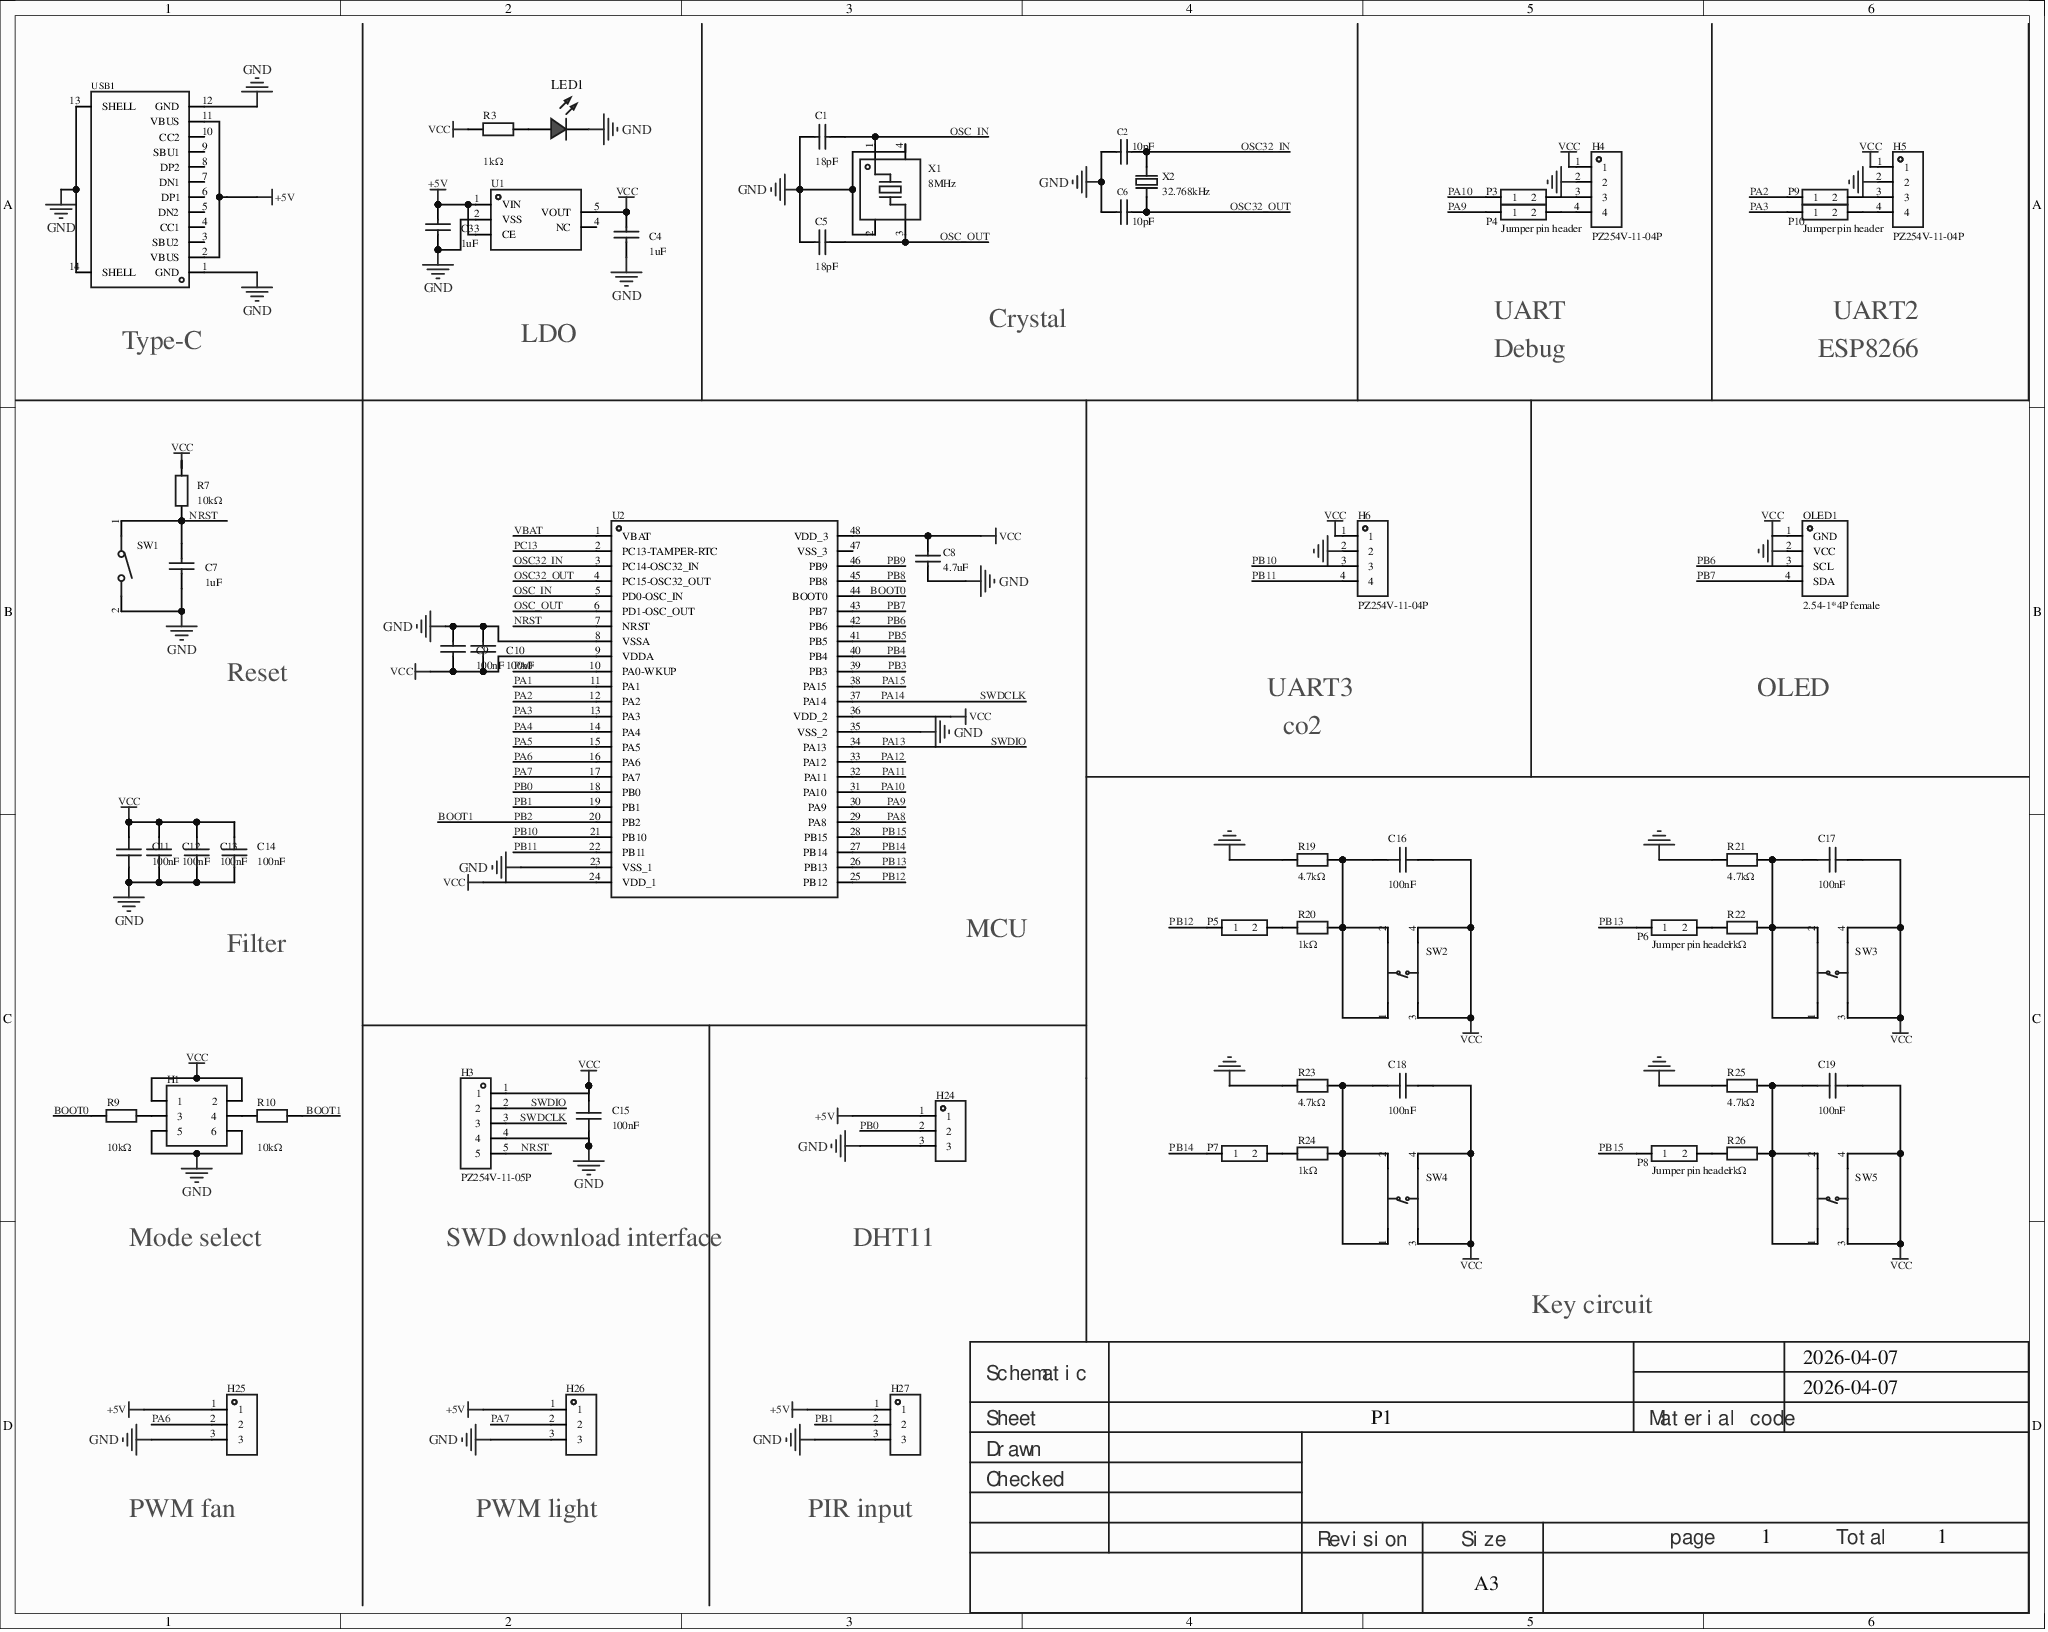
[diagram p0: MISC61607-3.schdoc]
# Altium project MISC61607-2.PrjPcb
1 sheet, 60 parts. Net scope: global (net labels, ports and power ports of the same name join across sheets).
Board file: MISC61607.pcbdoc

## Sheet MISC61607-3.schdoc
size 344 x 274 mm; Version: V1.0; @Project Name: MISC61607; @Page Count: 1; @Update Date: 2026-04-07; @Create Date: 2026-04-07; @Schematic Name: MISC61607; @Page No: 1; @Board Name: MISC61607; @Create Time: 19:36:59; @Update Time: 19:36:59

### Parts
C1  value 18pF  [C0603]  (hidden comment: FCC0603N180J500CT)
C2  value 10pF  [C0603]  (hidden comment: CL10C100JB8NNNC)
C3  value 1uF  [C0603]  (hidden comment: CL05A105KP5NNNC)
C4  value 1uF  [C0603]  (hidden comment: CL05A105KQ5NNNC)
C5  value 18pF  [C0603]  (hidden comment: FCC0603N180J500CT)
C6  value 10pF  [C0603]  (hidden comment: CL10C100JB8NNNC)
C7  value 1uF  [C0603]  (hidden comment: CGA0603X5R105K500JT)
C8  value 4.7uF  [C0603]  (hidden comment: CL10A475KO8NNNC)
C9  value 100nF  [C0603]  (hidden comment: CC0603KRX7R9BB104)
C10  value 100nF  [C0603]  (hidden comment: CC0603KRX7R9BB104)
C11  value 100nF  [C0603]  (hidden comment: CC0603KRX7R9BB104)
C12  value 100nF  [C0603]  (hidden comment: CC0603KRX7R9BB104)
C13  value 100nF  [C0603]  (hidden comment: CC0603KRX7R9BB104)
C14  value 100nF  [C0603]  (hidden comment: CC0603KRX7R9BB104)
C15  value 100nF  [C0603]  (hidden comment: CC0603KRX7R9BB104)
C16  100nF  [C0603]
C17  100nF  [C0603]
C18  100nF  [C0603]
C19  100nF  [C0603]
H1  (no value)  [HDR-TH_6P-P2.54-V-R2-C3-S2.54_A2541WV-2X3P]
H3  PZ254V-11-05P  [HDR-TH_5P-P2.54-V-M]
H4  PZ254V-11-04P  [HDR-TH_4P-P2.54-V-M]
H5  PZ254V-11-04P  [HDR-TH_4P-P2.54-V-M]
H6  PZ254V-11-04P  [HDR-TH_4P-P2.54-V-M]
H24  HC-PM254-8.5H-1x3PW-02A  [HDR-TH_3P-P2.54_HC-PM254-8.5H-1X3PW]  (value not drawn)
H25  HC-PM254-8.5H-1x3PW-02A  [HDR-TH_3P-P2.54_HC-PM254-8.5H-1X3PW]  (value not drawn)
H26  HC-PM254-8.5H-1x3PW-02A  [HDR-TH_3P-P2.54_HC-PM254-8.5H-1X3PW]  (value not drawn)
H27  HC-PM254-8.5H-1x3PW-02A  [HDR-TH_3P-P2.54_HC-PM254-8.5H-1X3PW]  (value not drawn)
LED1  LED_0402-R  [LED_0402]  (value not drawn)
OLED1  2.54-1*4P female  [HDR-TH_4P-P2.54-V-F]
P3  Jumper pin header  [2P排针]  (value not drawn)
P4  Jumper pin header  [2P排针]
P5  Jumper pin header  [2P排针]  (value not drawn)
P6  Jumper pin header  [2P排针]
P7  Jumper pin header  [2P排针]  (value not drawn)
P8  Jumper pin header  [2P排针]
P9  Jumper pin header  [2P排针]  (value not drawn)
P10  Jumper pin header  [2P排针]
R3  value 1kΩ  [R0603]  (hidden comment: 0603WAF1001T5E)
R7  value 10kΩ  [R0603]  (hidden comment: 0603WAF1002T5E)
R9  value 10kΩ  [R0603]  (hidden comment: 0603WAF1002T5E)
R10  value 10kΩ  [R0603]  (hidden comment: 0603WAF1002T5E)
R19  4.7kΩ  [R0603]
R20  1kΩ  [R0603]
R21  4.7kΩ  [R0603]
R22  1kΩ  [R0603]
R23  4.7kΩ  [R0603]
R24  1kΩ  [R0603]
R25  4.7kΩ  [R0603]
R26  1kΩ  [R0603]
SW1  TS-1088-AR02016  [SW-SMD_L3.9-W3.0-P4.45]  (value not drawn)
SW2  TS665CJ  [SW-TH_4P-L6.0-W6.0-P4.50-LS6.5]  (value not drawn)
SW3  TS665CJ  [SW-TH_4P-L6.0-W6.0-P4.50-LS6.5]  (value not drawn)
SW4  TS665CJ  [SW-TH_4P-L6.0-W6.0-P4.50-LS6.5]  (value not drawn)
SW5  TS665CJ  [SW-TH_4P-L6.0-W6.0-P4.50-LS6.5]  (value not drawn)
U1  ME6211C33M5G-N  [SOT-23-5_L3.0-W1.7-P0.95-LS2.8-BL]  (value not drawn)
U2  STM32F103C8T6  [LQFP-48_L7.0-W7.0-P0.50-LS9.0-BL]  (value not drawn)
USB1  TYPE-C 16PIN 2MD(073)  [USB-C-SMD_TYPE-C-6PIN-2MD-073]  (value not drawn)
X1  8MHz  [OSC-SMD_4P-L3.2-W2.5-BL]
X2  value 32.768kHz  [CRYSTAL-SMD_L3.2-W1.5-1]  (hidden comment: Q13FC13500049)

### Nets
+5V: C3.2 H24.1 H25.1 H26.1 H27.1 U1.1(VIN) U1.3(CE) USB1.2(VBUS) USB1.11(VBUS)
GND: C1.2 C2.1 C3.1 C4.1 C5.2 C6.1 C7.2 C8.1 C9.2 C10.2 C11.1 C12.1 C13.1 C14.1 C15.1 H1.5 H1.6 H3.4 H4.2 H5.2 H6.2 H24.3 H25.3 H26.3 H27.3 LED1.1(C) OLED1.2(VCC) R19.1 R21.1 R23.1 R25.1 SW1.2 U1.2(VSS) U2.8(VSSA) U2.23(VSS_1) U2.35(VSS_2) USB1.1(GND) USB1.12(GND) USB1.13(SHELL) USB1.14(SHELL) X1.2(GND) X1.4(GND)
VCC: C4.2 C8.2 C9.1 C10.1 C11.2 C12.2 C13.2 C14.2 C15.2 C16.2 C17.2 C18.2 C19.2 H1.1 H1.2 H3.1 H4.1 H5.1 H6.1 OLED1.1(GND) R3.1 R7.2 SW2.3(C) SW2.4(D) SW3.3(C) SW3.4(D) SW4.3(C) SW4.4(D) SW5.3(C) SW5.4(D) U1.5(VOUT) U2.9(VDDA) U2.24(VDD_1) U2.36(VDD_2) U2.48(VDD_3)
BOOT0: R9.1 U2.44(BOOT0)
BOOT1: R10.2 U2.20(PB2)  [also labelled PB2]
NRST: C7.1 H3.5 R7.1 SW1.1 U2.7(NRST)
OSC32_IN: C2.2 U2.3(PC14-OSC32_IN) X2.2
OSC32_OUT: C6.2 U2.4(PC15-OSC32_OUT) X2.1
OSC_IN: C1.1 U2.5(PD0-OSC_IN) X1.1
OSC_OUT: C5.1 U2.6(PD1-OSC_OUT) X1.3
PA0: U2.10(PA0-WKUP)
PA1: U2.11(PA1)
PA2: P9.1 U2.12(PA2)
PA3: P10.1 U2.13(PA3)
PA4: U2.14(PA4)
PA5: U2.15(PA5)
PA6: H25.2 U2.16(PA6)
PA7: H26.2 U2.17(PA7)
PA8: U2.29(PA8)
PA9: P4.1 U2.30(PA9)
PA10: P3.1 U2.31(PA10)
PA11: U2.32(PA11)
PA12: U2.33(PA12)
PA13: H3.2 U2.34(PA13)  [also labelled SWDIO]
PA14: H3.3 U2.37(PA14)  [also labelled SWDCLK]
PA15: U2.38(PA15)
PB0: H24.2 U2.18(PB0)
PB1: H27.2 U2.19(PB1)
PB3: U2.39(PB3)
PB4: U2.40(PB4)
PB5: U2.41(PB5)
PB6: OLED1.3(SCL) U2.42(PB6)
PB7: OLED1.4(SDA) U2.43(PB7)
PB8: U2.45(PB8)
PB9: U2.46(PB9)
PB10: H6.3 U2.21(PB10)
PB11: H6.4 U2.22(PB11)
PB12: P5.1 U2.25(PB12)
PB13: P6.1 U2.26(PB13)
PB14: P7.1 U2.27(PB14)
PB15: P8.1 U2.28(PB15)
PC13: U2.2(PC13-TAMPER-RTC)
VBAT: U2.1(VBAT)
NetC16_1: C16.1 R19.2 R20.2 SW2.1(A) SW2.2(B)
NetC17_1: C17.1 R21.2 R22.2 SW3.1(A) SW3.2(B)
NetC18_1: C18.1 R23.2 R24.2 SW4.1(A) SW4.2(B)
NetC19_1: C19.1 R25.2 R26.2 SW5.1(A) SW5.2(B)
NetH1_3: H1.3 R9.2
NetH1_4: H1.4 R10.1
NetH4_3: H4.3 P3.2
NetH4_4: H4.4 P4.2
NetH5_3: H5.3 P9.2
NetH5_4: H5.4 P10.2
NetLED1_2: LED1.2(A) R3.2
NetP5_2: P5.2 R20.1
NetP6_2: P6.2 R22.1
NetP7_2: P7.2 R24.1
NetP8_2: P8.2 R26.1

Not connected (* = marked no-connect by the designer): U1 4(NC)*; U2 47(VSS_3); USB1 3(SBU2)* 4(CC1) 5(DN2) 6(DP1) 7(DN1) 8(DP2) 9(SBU1)* 10(CC2)

### Notes on the sheet
- (near USB1) Type-C
- LDO
- Crystal
- UART
- Debug
- ESP8266
- UART2
- Reset
- UART3
- co2
- OLED
- Filter
- MCU
- Mode select
- SWD download interface
- DHT11
- Key circuit
- (near H25) PWM fan
- (near H26) PWM light
- (near H27) PIR input
- 2026-04-07
- Schematic
- Sheet
- P1
- Material code
- Checked
- Drawn
- Revision
- Size
- A3
- page
- 1
- Total

### Library data of the parts
C1 C5 = FCC0603N180J500CT: Capacitance:18pF; tolerance:±5%; rated voltage:50V; temperature coefficient:C0G;; Manufacturer: FOJAN(富捷); Symbol: 0402CG180J500NT; AddInBom: yes; ModelId: ac125912035d415993ca9572d50418b1; ModelName: C0603_L1.6-W0.8-H0.8; ModelTransform: 62.992,31.496,0,0,0,0,0,0,0; Tolerance: ±5%; Voltage Rating: 50V; Temperature Coefficient: C0G; Device: FCC0603N180J500CT; Supplier: LCSC; Manufacturer Part: FCC0603N180J500CT; Supplier Part: C5137620; JLCPCB Part Class: Extended Part; LCSC Part Name: 18pF ±5% 50V; Supplier Footprint: 0603; Datasheet: https://atta.szlcsc.com/upload/public/pdf/source/20220818/0EB3B7FB2F5648AC16609637FBA7DABE.pdf; ConvertToPcb: yes; FootprintName: C0603
C2 C6 = CL10C100JB8NNNC: Capacitance:10pF; tolerance:±5%; rated voltage:50V; temperature coefficient:C0G;; Manufacturer: SAMSUNG(三星); Symbol: 0402CG100J500NT; AddInBom: yes; ModelId: ac125912035d415993ca9572d50418b1; ModelName: C0603_L1.6-W0.8-H0.8; ModelTransform: 62.992,31.496,0,0,0,0,0,0,0; Tolerance: ±5%; Voltage Rating: 50V; Temperature Coefficient: C0G; Device: CL10C100JB8NNNC; Supplier: LCSC; Manufacturer Part: CL10C100JB8NNNC; Capacitance: 10pF; Supplier Part: C1634; JLCPCB Part Class: Basic Part; LCSC Part Name: 10pF ±5% 50V; Supplier Footprint: 0603; Datasheet: https://item.szlcsc.com/datasheet/CL10C100JB8NNNC/1986.html; ConvertToPcb: yes; FootprintName: C0603
C3 = CL05A105KP5NNNC: Capacitance:1uF; tolerance:±10%; rated voltage:10V; dielectric (temperature coefficient):X5R;; Manufacturer: SAMSUNG(三星); AddInBom: yes; ModelId: 36a51122f27c49738f86b3bfa98863e0; ModelName: C0402_L1.0-W0.5-H0.5; ModelTransform: 39.37,19.685,0,0,0,0,0,0,0; Tolerance: ±10%; Voltage Rated: 10V; Temperature Coefficient: X5R; Symbol: CL05A105KP5NNNC; Device: CL05A105KP5NNNC; Supplier: LCSC; Manufacturer Part: CL05A105KP5NNNC; Supplier Part: C14445; JLCPCB Part Class: Extended library; LCSC Part Name: 1uF ±10% 10V; Supplier Footprint: 0402; Datasheet: https://atta.szlcsc.com/upload/public/pdf/source/20160218/1457707763339.pdf; ConvertToPcb: yes; FootprintName: C0603
C4 = CL05A105KQ5NNNC: Capacitance:1uF; tolerance:±10%; rated voltage:6.3V; dielectric (temperature coefficient):X5R;; Manufacturer: SAMSUNG(三星); AddInBom: yes; ModelId: 36a51122f27c49738f86b3bfa98863e0; ModelName: C0402_L1.0-W0.5-H0.5; ModelTransform: 39.37,19.685,0,0,0,0,0,0,0; Tolerance: ±10%; Voltage Rated: 6.3V; Temperature Coefficient: X5R; Symbol: CL05A105KQ5NNNC; Device: CL05A105KQ5NNNC; Supplier: LCSC; Manufacturer Part: CL05A105KQ5NNNC; Supplier Part: C107372; JLCPCB Part Class: Extended library; LCSC Part Name: 1uF ±10% 6.3V; Supplier Footprint: 0402; Datasheet: https://atta.szlcsc.com/upload/public/pdf/source/20160218/1457707763339.pdf; ConvertToPcb: yes; FootprintName: C0603
C7 = CGA0603X5R105K500JT: Capacitance:1uF; tolerance:±10%; rated voltage:50V; temperature coefficient:X5R;; Manufacturer: HRE(芯声); Symbol: CL05A105KQ5NNNC; AddInBom: yes; ModelId: ac125912035d415993ca9572d50418b1; ModelName: C0603_L1.6-W0.8-H0.8; ModelTransform: 62.992,31.496,0,0,0,0,0,0,0; Tolerance: ±10%; Voltage Rating: 50V; Temperature Coefficient: X5R; Device: CGA0603X5R105K500JT; Supplier: LCSC; Manufacturer Part: CGA0603X5R105K500JT; Supplier Part: C6119852; JLCPCB Part Class: Extended Part; LCSC Part Name: 1uF ±10% 50V; Supplier Footprint: 0603; ConvertToPcb: yes; FootprintName: C0603
C8 = CL10A475KO8NNNC: Capacitance:4.7uF; tolerance:±10%; rated voltage:16V; temperature coefficient:X5R;; Manufacturer: SAMSUNG(三星); Symbol: CL05A475MP5NRNC; AddInBom: yes; ModelId: ac125912035d415993ca9572d50418b1; ModelName: C0603_L1.6-W0.8-H0.8; ModelTransform: 62.992,31.496,0,0,0,0,0,0,0; Tolerance: ±10%; Voltage Rating: 16V; Temperature Coefficient: X5R; Device: CL10A475KO8NNNC; Supplier: LCSC; Manufacturer Part: CL10A475KO8NNNC; Supplier Part: C19666; JLCPCB Part Class: Basic Part; LCSC Part Name: 4.7uF ±10% 16V; Supplier Footprint: 0603; Datasheet: https://item.szlcsc.com/datasheet/CL10A475KO8NNNC/20375.html; ConvertToPcb: yes; FootprintName: C0603
C9 = CC0603KRX7R9BB104: Capacitance:100nF; tolerance:±10%; rated voltage:50V; temperature coefficient:X7R;; Manufacturer: YAGEO(国巨); Symbol: CC0402KRX7R9BB103; AddInBom: yes; ModelId: ac125912035d415993ca9572d50418b1; ModelName: C0603_L1.6-W0.8-H0.8; ModelTransform: 62.992,31.496,0,0,0,0,0,0,0; Tolerance: ±10%; Voltage Rating: 50V; Temperature Coefficient: X7R; Device: CC0603KRX7R9BB104; Supplier: LCSC; Manufacturer Part: CC0603KRX7R9BB104; Supplier Part: C14663; JLCPCB Part Class: Basic Part; LCSC Part Name: 100nF ±10% 50V; Supplier Footprint: 0603; Datasheet: https://item.szlcsc.com/datasheet/CC0603KRX7R9BB104/15331.html; ConvertToPcb: yes; FootprintName: C0603
C10 = CC0603KRX7R9BB104: Capacitance:100nF; tolerance:±10%; rated voltage:50V; temperature coefficient:X7R;; Manufacturer: YAGEO(国巨); Symbol: CL05A105KP5NNNC; AddInBom: yes; ModelId: ac125912035d415993ca9572d50418b1; ModelName: C0603_L1.6-W0.8-H0.8; ModelTransform: 62.992,31.496,0,0,0,0,0,0,0; Tolerance: ±10%; Voltage Rating: 50V; Temperature Coefficient: X7R; Device: CC0603KRX7R9BB104; Supplier: LCSC; Manufacturer Part: CC0603KRX7R9BB104; Supplier Part: C14663; JLCPCB Part Class: Basic Part; LCSC Part Name: 100nF ±10% 50V; Supplier Footprint: 0603; Datasheet: https://item.szlcsc.com/datasheet/CC0603KRX7R9BB104/15331.html; ConvertToPcb: yes; FootprintName: C0603
C11-C15 = CC0603KRX7R9BB104: Capacitance:100nF; tolerance:±10%; rated voltage:50V; temperature coefficient:X7R;; Manufacturer: YAGEO(国巨); Symbol: CC0402KRX7R7BB104; AddInBom: yes; ModelId: ac125912035d415993ca9572d50418b1; ModelName: C0603_L1.6-W0.8-H0.8; ModelTransform: 62.992,31.496,0,0,0,0,0,0,0; Tolerance: ±10%; Voltage Rating: 50V; Temperature Coefficient: X7R; Device: CC0603KRX7R9BB104; Supplier: LCSC; Manufacturer Part: CC0603KRX7R9BB104; Supplier Part: C14663; JLCPCB Part Class: Basic Part; LCSC Part Name: 100nF ±10% 50V; Supplier Footprint: 0603; Datasheet: https://item.szlcsc.com/datasheet/CC0603KRX7R9BB104/15331.html; ConvertToPcb: yes; FootprintName: C0603
C16-C19 = CGA0603X7R104K500JT: Capacitance:100nF; tolerance:±10%; rated voltage:50V; temperature coefficient:X7R;; Manufacturer: HRE(芯声); AddInBom: yes; ModelId: ac125912035d415993ca9572d50418b1; ModelName: C0603_L1.6-W0.8-H0.8; ModelTransform: 62.992,31.496,0,0,0,0,0,0,0; Tolerance: ±10%; Voltage Rating: 50V; Temperature Coefficient: X7R; Symbol: CGA0603X7R104K500JT; Device: CGA0603X7R104K500JT; LCSC Part Name: 100nF ±10% 50V; SupplierPart: C6119867; ManufacturerPart: CGA0603X7R104K500JT; Supplier Footprint: 0603; Datasheet: https://atta.szlcsc.com/upload/public/pdf/source/20250103/C44077DA9E7B3EFAE02F22B6D3D1CBC9.pdf; Supplier: LCSC; ConvertToPcb: yes; FootprintName: C0603; Value: 100nF
H1 = HDR-M_2.54_2x3: Symbol: HDR-M-2.54_2x3; ConvertToPcb: yes; ModelId: fd1b55b786fb415ca65c4187088147b7; ModelName: HDR2.54-M-LI-2x3P; ModelTransform: 299.9994,200,0,0,0,0,0,0,-118.11; Device: HDR-M_2.54_2x3; AddInBom: yes; SupplierPart: C402781; Supplier Footprint: 插件,P=2.54mm; FootprintName: HDR-TH_6P-P2.54-V-R2-C3-S2.54_A2541WV-2X3P
H3 = PZ254V-11-05P: Pin structure:1x5P; pitch:2.54mm; row spacing:-; round/square pin:square pin; mounting:through-hole; rows:single row; total PIN count:5P; rated current:-; rated voltage:-; mating pin length:6mm; plastic height:2.5mm; tail length:3mm; contact material:brass; contact plating:-; operating temperature:-40℃~+105℃; colour:black;; Manufacturer: XFCN(兴飞); AddInBom: yes; ModelId: 47d466e4a34f4fc5bc626cf773a24dd5; ModelName: HDR-TH_5P-P2.54-M-LI-1X5P; ModelTransform: 499.999,100,0,0,0,0,0,0,-118.11; Pin Structure: 1x5P; Pitch: 2.54mm; Symbol: PZ254V-11-05P; Device: PZ254V-11-05P; LCSC Part Name: 1x5P 间距:2.54mm 方针 直插; SupplierPart: C492404; ManufacturerPart: PZ254V-11-05P; Supplier Footprint: 插件,P=2.54mm; JLCPCB Part Class: Extended library; Datasheet: https://atta.szlcsc.com/upload/public/pdf/source/20200309/C492404_E51533260F8710EFF5D4617281164C1D.pdf; Supplier: LCSC; ConvertToPcb: yes; FootprintName: HDR-TH_5P-P2.54-V-M; Row Spacing: -; Circluar Pins/Square Pins: Square pin; Mounting Type: Through-hole; Number of Rows: Single row; Number of Pins: 5P; Current Rating: -; Voltage Rating (Max): -; Length of Mating Pin: 6mm; Insulation Height: 2.5mm; Length of End Connection Pin: 3mm; Contact Material: Brass; Contact Plating: -; Operating Temperature: -40℃~+105℃; Color: Black
H4-H6 = PZ254V-11-04P: Pin structure:1x4P; pitch:2.54mm; row spacing:-; round/square pin:square pin; mounting:through-hole; rows:single row; total PIN count:4P; rated current:3A; rated voltage:250V; mating pin length:6mm; plastic height:2.5mm; tail length:3mm; contact material:-; operating temperature:-40℃~+105℃; colour:black;; Manufacturer: XFCN(兴飞); Symbol: PZ254V-11-04P_C2691448; AddInBom: yes; ModelId: 112f4d05e8d64e99ab9a333894bea4f9; ModelName: HDR-TH_4P-P2.54-M-LI-1X4P; ModelTransform: 399.999,104.7242,0,0,0,0,0,0,-118.11; Pin Structure: 1x4P; Pitch: 2.54mm; Current Rating: 3A; Voltage Rating (Max): 250V; Device: PZ254V-11-04P; LCSC Part Name: 1x4P 间距:2.54mm 方针 直插; SupplierPart: C2691448; ManufacturerPart: PZ254V-11-04P; Supplier Footprint: 插件,P=2.54mm; JLCPCB Part Class: Extended library; Datasheet: https://item.szlcsc.com/datasheet/PZ254V-11-04P/2801085.html; Supplier: LCSC; ConvertToPcb: yes; FootprintName: HDR-TH_4P-P2.54-V-M; Row Spacing: -; Circluar Pins/Square Pins: Square pin; Mounting Type: Through-hole; Number of Rows: Single row; Number of Pins: 4P; Length of Mating Pin: 6mm; Insulation Height: 2.5mm; Length of End Connection Pin: 3mm; Contact Material: -; Operating Temperature: -40℃~+105℃; Color: Black
H24-H27 = HC-PM254-8.5H-1x3PW-02A: Socket structure:1x3P; pitch:2.54mm; row spacing:-; round/square hole:square hole; mounting:bent (right-angle); rows:single row; total hole count:3P; rated current:3A; rated voltage:-; socket direction:side; plastic height:2.5mm; contact material:brass; contact plating:gold; operating temperature:-40℃~+105℃;; Manufacturer: HC(虹成电子); AddInBom: yes; ModelId: e14a0b847ce14913bcceafd4aa6783c3; ModelTransform: 320.078,397.637,0,0,0,0,0,-194.133,-125.984; Holes Structure: 1x3P; Pitch: 2.54mm; Number of Positions: 3P; Current Rating: 3A; Holes Direction: Side; PIN Length: 3mm; Symbol: HC-PM254-8.5H-1X3PW; Device: HC-PM254-8.5H-1x3PW-02A; LCSC Part Name: 间距2.54mm 1x3Pin 弯插 PC3.2 PB10.2 H8.5; SupplierPart: C22373927; ManufacturerPart: HC-PM254-8.5H-1x3PW-02A; Supplier Footprint: 弯插,P=2.54mm; Datasheet: https://atta.szlcsc.com/upload/public/pdf/source/20250106/76C6231410311B19092B3A33DDCC33AF.pdf; Supplier: LCSC; ConvertToPcb: yes; FootprintName: HDR-TH_3P-P2.54_HC-PM254-8.5H-1X3PW; ModelName: HDR-TH_3P-P2.54_HC-PM254-8.5H-1X3PW; Row Spacing: -; Circular Hole / Square Hole: Square hole; Mounting Type: Bent (right-angle); Number of Rows: Single row; Voltage Rating (Max): -; Insulation Height: 2.5mm; Contact Material: Brass; Contact Plating: Gold; Operating Temperature: -40℃~+105℃; Supplementary Features: -
LED1 = LED_0402-R: Symbol: LED_R; Convert to PCB: yes; 3D Model: ff479c6f784e45d5abe8f8ff531b4a70; 3D Model Transform: 39.4,19.7,15.76,180,0,0,0,0,0; ModelName: LED0402-RD_ORANGE; Device: LED_0402-R; Add into BOM: yes; Supplier Footprint: 0402; FootprintName: LED_0402
OLED1 = 2.54-1*4P母: Socket structure:1x4P; pitch:2.54mm; row spacing:-; round/square hole:square hole; mounting:through-hole; rows:single row; total hole count:4P; rated current:3A; rated voltage:-; socket direction:top; plastic height:-; contact material:bronze; contact plating:-; operating temperature:-40℃~+105℃;; Manufacturer: BOOMELE(博穆精密); Symbol: HS96L03W2C03; AddInBom: yes; ModelId: d187812051054f85879fcaa51a310d8e; ModelTransform: 419.6842,98.464,0,0,0,0,0,0,-118.11; Holes Structure: 1x4P; Pitch: 2.54mm; Number of Positions: 4P; Current Rating: 3A; Holes Direction: Top; Device: 2.54-1*4P female; LCSC Part Name: 间距:2.54mm 1x4P 直插; SupplierPart: C2718488; ManufacturerPart: 2.54-1*4P母; Supplier Footprint: 插件,P=2.54mm; JLCPCB Part Class: Extended Part; Datasheet: https://item.szlcsc.com/datasheet/2.54-1*4P%25E6%25AF%258D/2834502.html; Supplier: LCSC; ConvertToPcb: yes; FootprintName: HDR-TH_4P-P2.54-V-F; ModelName: HDR-TH_4P-P2.54-V-F; Row Spacing: -; Circular Hole / Square Hole: Square hole; Mounting Type: Through-hole; Number of Rows: Single row; Voltage Rating (Max): -; Insulation Height: -; Contact Material: Bronze; Contact Plating: -; Operating Temperature: -40℃~+105℃
P3-P10 = 跳线排针-1.27mm-1×2P: AddInBom: yes; Device: 跳线排针-1.27mm-1×2P; 物料号: *; 名称: Jumper pin header; 封装: 1.27mm-1×2P; 规格: 1.27mm-1×2P; 型号: *; 替换型号: *; 厂商: *; Footprint Name: 跳线排针-1.27mm-1×2P; ConvertToPcb: yes; SymbolName: 跳线排针-1.27mm-1×2P
R3 = 0603WAF1001T5E: Resistor type:thick film resistor; resistance:1kΩ; tolerance:±1%; power:100mW; max working voltage:75V; temperature coefficient:±100ppm/℃;; Manufacturer: UNI-ROYAL(厚声); Symbol: 0402WGF1001TCE; AddInBom: yes; ModelId: fc143cca1e79419f9cd78b61e9279f08; ModelTransform: 31.8897,63.7794,0,90,0,0,0,0,0; Tolerance: ±1%; Power(Watts): 100mW; Overload Voltage (Max): 75V; JLCPCB Part Class: Basic Part; Device: 0603WAF1001T5E; Supplier: LCSC; Manufacturer Part: 0603WAF1001T5E; Supplier Part: C21190; LCSC Part Name: 1kΩ ±1% 100mW 厚膜电阻; Supplier Footprint: 0603; Datasheet: https://atta.szlcsc.com/upload/public/pdf/source/20200306/C422600_1E6D84923E4A46A82E41ADD87F860B5C.pdf; ConvertToPcb: yes; FootprintName: R0603; ModelName: R0603; Type: Thick film resistor; Temperature Coefficient: ±100ppm/℃; Operating Temperature Range: -55℃~+155℃
R7 R9 R10 = 0603WAF1002T5E: Resistor type:thick film resistor; resistance:10kΩ; tolerance:±1%; power:100mW; working voltage:75V; temperature coefficient:±100ppm/℃;; Manufacturer: UNI-ROYAL(厚声); Symbol: RC0402FR-0710KL; AddInBom: yes; ModelId: fc143cca1e79419f9cd78b61e9279f08; ModelTransform: 31.8897,63.7794,0,90,0,0,0,0,0; Tolerance: ±1%; Power(Watts): 100mW; Voltage-Supply(Max): 75V; Device: 0603WAF1002T5E; LCSC Part Name: 厚膜电阻 10kΩ ±1% 100mW; SupplierPart: C25804; ManufacturerPart: 0603WAF1002T5E; Supplier Footprint: 0603; JLCPCB Part Class: Basic Part; Datasheet: https://item.szlcsc.com/datasheet/0603WAF1002T5E/26547.html; Supplier: LCSC; ConvertToPcb: yes; FootprintName: R0603; ModelName: R0603; Type: Thick film resistor; Temperature Coefficient: ±100ppm/℃; Operating Temperature: -55℃~+155℃
R19 R21 R23 R25 = 0603WAF4701T5E: Resistor type:thick film resistor; resistance:4.7kΩ; tolerance:±1%; power:100mW; working voltage:75V; temperature coefficient:±100ppm/℃;; Manufacturer: UNI-ROYAL(厚声); AddInBom: yes; ModelId: fc143cca1e79419f9cd78b61e9279f08; ModelTransform: 31.8897,63.7794,0,90,0,0,0,0,0; Tolerance: ±1%; Power(Watts): 100mW; Voltage-Supply(Max): 75V; Symbol: 0603WAF4701T5E; Device: 0603WAF4701T5E; LCSC Part Name: 4.7kΩ ±1% 100mW 厚膜电阻; SupplierPart: C23162; ManufacturerPart: 0603WAF4701T5E; Supplier Footprint: 0603; Datasheet: https://item.szlcsc.com/datasheet/0603WAF4701T5E/23889.html; Supplier: LCSC; ConvertToPcb: yes; FootprintName: R0603; ModelName: R0603; Type: Thick film resistor; Value: 4.7kΩ; Temperature Coefficient: ±100ppm/℃; Operating Temperature: -55℃~+155℃
R20 R22 R24 R26 = 0603WAF1001T5E: Resistor type:thick film resistor; resistance:1kΩ; tolerance:±1%; power:100mW; max working voltage:75V; temperature coefficient:±100ppm/℃;; Manufacturer: UNI-ROYAL(厚声); AddInBom: yes; ModelId: fc143cca1e79419f9cd78b61e9279f08; ModelTransform: 31.8897,63.7794,0,90,0,0,0,0,0; Tolerance: ±1%; Power(Watts): 100mW; Overload Voltage (Max): 75V; Symbol: 0603WAF1001T5E; Device: 0603WAF1001T5E; LCSC Part Name: 1kΩ ±1% 100mW 厚膜电阻; SupplierPart: C21190; ManufacturerPart: 0603WAF1001T5E; Supplier Footprint: 0603; JLCPCB Part Class: Basic library; Datasheet: https://atta.szlcsc.com/upload/public/pdf/source/20200306/C422600_1E6D84923E4A46A82E41ADD87F860B5C.pdf; Supplier: LCSC; ConvertToPcb: yes; FootprintName: R0603; ModelName: R0603; Type: Thick film resistor; Value: 1kΩ; Temperature Coefficient: ±100ppm/℃; Operating Temperature Range: -55℃~+155℃
SW1 = TS-1088-AR02016: Contact current:50mA; rated voltage (DC):12V; insulation resistance:100MΩ; circuit:SPST; mounting:vertical SMD; actuation force:160gf@±50gf; mechanical life:10万 cycles; with bracket:no;; Manufacturer: XUNPU(讯普); AddInBom: yes; ModelId: b26698b69f274ffabef8a26c7d0e5dd1; ModelName: SW-SMD_L3.9-W2.9-H2.0-LS4.8; ModelTransform: 188.976,114.174,0,0,0,0,0,0,0; Contact Current: 50mA; Voltage Rating (DC): 12V; Insulation Resistance: 100MΩ; Circuit: SPST; Actuator Style: Round button; Actuator/Cap Color: Black; Pin Style: SMD tab; Switch Length: 4mm; Switch Width: 3mm; Switch Height: 2mm; Strike Gundam: No; Device: TS-1088-AR02016; Symbol: TS-1088-AR02016; LCSC Part Name: 4*3*2mm 立贴 轻触开关; SupplierPart: C720477; ManufacturerPart: TS-1088-AR02016; Supplier Footprint: SMD; JLCPCB Part Class: Extended library; Datasheet: https://atta.szlcsc.com/upload/public/pdf/source/20200810/C720475_60D09DD6C54279ADDB2DC25100F1CC11.pdf; Supplier: LCSC; ConvertToPcb: yes; FootprintName: SW-SMD_L3.9-W3.0-P4.45; Mounting Style: Vertical SMD; Operating Force: 160gf@±50gf; Mechanical Life: 10万 cycles; Operating Temperature: -30℃~+80℃
SW2-SW5 = TS665CJ: Circuit:SPST; button shape:round button; mounting:through-hole; switch length:6mm; switch width:6mm; switch height:5mm; contact current:50mA; rated voltage (DC):12V; with light:-; mechanical life:-;; Manufacturer: SHOU HAN(首韩); AddInBom: yes; ModelId: 20eee248bc684ccd8cbdbb1d0d91ec6f; ModelName: SW-TH_4P-L6.0-W6.0-H5.0-LS6.5-P4.50; ModelTransform: 236.22,323.03,0,90,0,0,0,0,-137.795; Circuit: SPST; Switch Length: 6mm; Switch Height: 5mm; Contact Current: 50mA; Voltage Rating (DC): 12V; Symbol: TS665CJ; Device: TS665CJ; LCSC Part Name: 6*6*5mm 直插 轻触开关; SupplierPart: C393938; ManufacturerPart: TS665CJ; Supplier Footprint: 插件; JLCPCB Part Class: Extended library; Datasheet: https://atta.szlcsc.com/upload/public/pdf/source/20190521/C393938_BDABEAC600B4C55E200A80AA129B70BC.pdf; Supplier: LCSC; ConvertToPcb: yes; FootprintName: SW-TH_4P-L6.0-W6.0-P4.50-LS6.5; Actuator Style: Round button; Mounting Style: Through-hole; Switch Width: 6mm; With Lamp: -; Mechanical Life: -
U1 = ME6211C33M5G-N: Output type:fixed; output polarity:positive; max input voltage:6V; output voltage:3.3V; output current:500mA; PSRR:70dB;; Manufacturer: MICRONE(南京微盟); Symbol: me6211c25m5g; AddInBom: yes; ModelId: 0a2a1b8f50944f73965918ad6e5fe167; ModelName: SOT-23-5_L2.9-W1.6-H1.1-LS2.8-P0.95; ModelTransform: 118.60433,114.173,0,90,0,0,0.0005,0.0005,0; Output Type: Fixed; Number of Outputs: 1; Maximum Input Voltage: 6V; Output Voltage: 3.3V; Dropout Voltage: 260mV@(200mA); Output Current: 500mA; Power Supply Rejection Ratio (PSRR): 70dB; Device: ME6211C33M5G-N; LCSC Part Name: ME6211C33M5G-N; SupplierPart: C82942; ManufacturerPart: ME6211C33M5G-N; Supplier Footprint: SOT-23-5; JLCPCB Part Class: Extended Part; Datasheet: https://atta.szlcsc.com/upload/public/pdf/source/20170918/C82942_1505727073070976520.pdf; Supplier: LCSC; ConvertToPcb: yes; FootprintName: SOT-23-5_L3.0-W1.7-P0.95-LS2.8-BL; Output Polarity: Positive
U2 = STM32F103C8T6: CPU core:CM3; program memory:64KB; total RAM:20KB; GPIO count:37; operating voltage range:2V~3.6V; max CPU frequency:72MHz; program memory type:FLASH;; Manufacturer: ST(意法半导体); AddInBom: yes; ModelId: 093be70396ff421eb2cdb946d5311efc; ModelName: LQFP-48_L7.0-W7.0-H1.4-LS9.0-P0.50; ModelTransform: 354.331,354.331,0,0,0,0,0,0,0; CPU Core: CM3; Program Storage Size: 64KB; RAM Size: 20KB; GPIO Ports Number: 37; CPU Maximum Speed: 72MHz; Program Memory Type: FLASH; ADC (Bit): 12bit; Peripheral/Function: Watchdog; DMA; Watchdog; on-chip temperature sensor; Symbol: STM32F103C8T6; Device: STM32F103C8T6; LCSC Part Name: STM32F103C8T6 MSL=3; SupplierPart: C8734; ManufacturerPart: STM32F103C8T6; Supplier Footprint: LQFP-48(7x7); JLCPCB Part Class: Extended library; Datasheet: https://atta.szlcsc.com/upload/public/pdf/source/20220812/8363ACEC51AD55ECEB84799464F7CB85.pdf; Supplier: LCSC; ConvertToPcb: yes; FootprintName: LQFP-48_L7.0-W7.0-P0.50-LS9.0-BL; Operating Voltage Range: 2V~3.6V; Operating Temperature Range: -40℃~+85℃; DAC (Bit): -; PWM (Bit): -; Universal Serial Bus: Yes; Internal Comparator: -; communication protocol: -; Watchdog: Yes; Real-Time Clock: -; Infrared Data Association: Yes; Low-Voltage Detect: Yes; CCP Capture/Compare: -; Secure Digital Input and Output: -; Direct Memory Access: Yes; Internal Oscillator: Yes
USB1 = TYPE-C 16PIN 2MD(073): Connector type:Type-C; standard:-; gender:female; contacts:16; ports:1; mounting:horizontal SMD; rated current - power:5A; operating temperature:-25℃~+85℃;; Manufacturer: SHOU HAN(首韩); AddInBom: yes; ModelId: 3a41b9ec9b654a0fad4d118405ec6290; ModelTransform: 351.9678,298.4246,0,0,0,0,0,-47.244,-35.433; Gender: Female; Number of Contacts: 16; Number of Ports: 1; Current Rating - Power (Max): 5A; Symbol: TYPE-C 16PIN 2MD(073); Device: TYPE-C 16PIN 2MD(073); Supplier: LCSC; Supplier Part: C2765186; Manufacturer Part: TYPE-C 16PIN 2MD(073); JLCPCB Part Class: Extended Part; LCSC Part Name: TYPE-C母座 16P 4脚插件带定位柱 不锈钢外壳 2次模顶; Supplier Footprint: SMD; ConvertToPcb: yes; FootprintName: USB-C-SMD_TYPE-C-6PIN-2MD-073; ModelName: USB-C-SMD_TYPE-C-6PIN-2MD-073; Connector Type: Type-C; Standard: -; Mounting Style: Horizontal SMD; Operating Temperature Range: -25℃~+85℃
X1 = X32258MOB4SI: Crystal type:SMD crystal; frequency:8MHz; room-temperature frequency tolerance:±10ppm; load capacitance:12pF; frequency stability (full temperature):±20ppm;; Manufacturer: YXC(扬兴晶振); AddInBom: yes; ModelId: ae22b8d143894765bc8100c37cb6356f; ModelName: OSC-SMD_4P-L3.2-W2.5-H1.0; ModelTransform: 125.984,98.425,0,0,0,0,0,0,0; Normal temperature Frequency Tolerance: ±10ppm; External load capacitor: 12pF; Frequency Stability(Full temperature range): ±20ppm; Equivalent Series Resistance (ESR): 150Ω; Symbol: X32258MOB4SI; Device: X32258MOB4SI; LCSC Part Name: 8MHz ±10ppm 12pF; SupplierPart: C2682775; ManufacturerPart: X32258MOB4SI; Supplier Footprint: SMD3225-4P; JLCPCB Part Class: Extended library; Datasheet: https://atta.szlcsc.com/upload/public/pdf/source/20240329/19D5F850207469550BEB00D7DFEDBC7A.pdf; Supplier: LCSC; ConvertToPcb: yes; FootprintName: OSC-SMD_4P-L3.2-W2.5-BL; Crystal Type: SMD crystal; Value: 8MHz; Operating Temperature: -40℃~+85℃
X2 = Q13FC13500049: Crystal type:SMD crystal; frequency:32.768kHz; room-temperature frequency tolerance:±20ppm; load capacitance:6pF;; Manufacturer: EPSON(爱普生); Symbol: Q13FC1350004900; AddInBom: yes; ModelId: 762d7afc596f4558a373612390f4386d; ModelTransform: 125.984,59.055,0,0,0,0,0,0,0; Normal temperature Frequency Tolerance: ±20ppm; External load capacitor: 6pF; Equivalent Series Resistance (ESR): 70kΩ; Device: Q13FC13500049; LCSC Part Name: 32.768kHz ±20ppm 6pF; SupplierPart: C95361; ManufacturerPart: Q13FC13500049; Supplier Footprint: SMD3215-2P; JLCPCB Part Class: Extended library; Datasheet: https://atta.szlcsc.com/upload/public/pdf/source/20230307/B34DAB909D91A4E9CF7EB9FB947CF9CB.pdf; Supplier: LCSC; ConvertToPcb: yes; FootprintName: CRYSTAL-SMD_L3.2-W1.5-1; ModelName: CRYSTAL-SMD_L3.2-W1.5-1; Crystal Type: SMD crystal; Operating Temperature: -40℃~+85℃